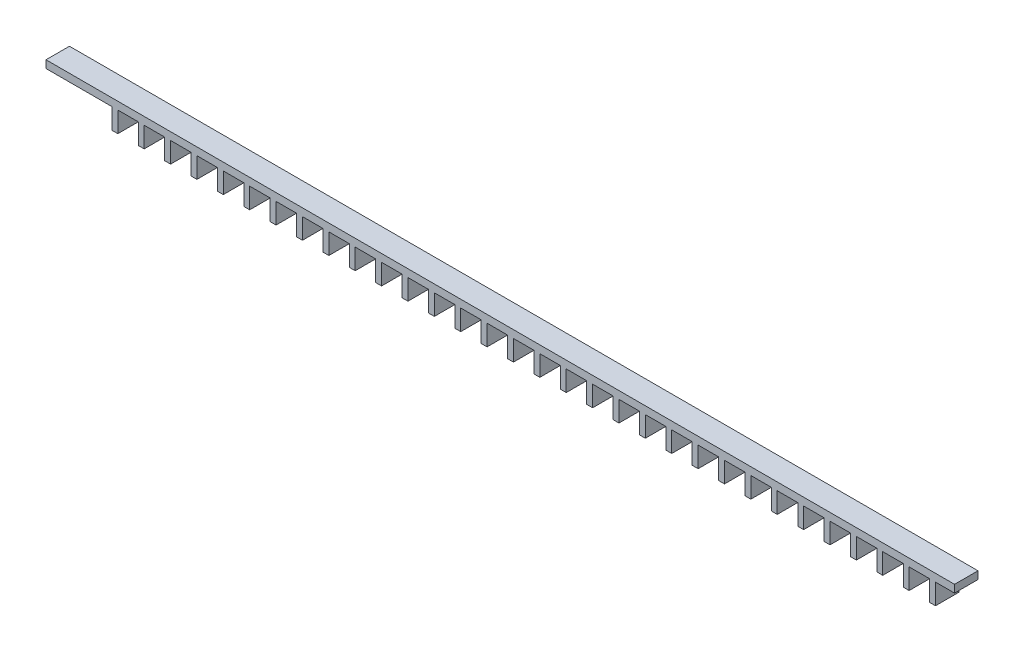
from build123d import *

# Parameters (mm, degrees)
SKETCH_1_W          = 1550
SKETCH_1_H          = 40
EXTRUDE_1_DEPTH     = 48
SKETCH_2_W          = 35
SKETCH_2_H          = 35
CUT_EXTRUDE_1_DEPTH = 778.514630087
SKETCH_6_W          = 35
SKETCH_6_H          = 35
CUT_EXTRUDE_5_DEPTH = 778.514630087
SKETCH_7_W          = 110
SKETCH_7_H          = 61.445783933
SKETCH_7_W_2        = 90
SKETCH_7_H_2        = 84.634966513
CUT_EXTRUDE_6_DEPTH = 778.514630087
SKETCH_8_W          = 40
SKETCH_8_H          = 13
EXTRUDE_2_DEPTH     = 10
SKETCH_9_W          = 40
SKETCH_9_H          = 13
CUT_EXTRUDE_7_DEPTH = 10
SKETCH_10_W         = 40
SKETCH_10_H         = 35
EXTRUDE_3_DEPTH     = 5
SKETCH_11_W         = 40
SKETCH_11_H         = 35
EXTRUDE_4_DEPTH     = 5
MOVE_FACE_1_BY      = 22.5
MOVE_FACE_1_2_BY    = 22.5
SKETCH_12_W         = 10
SKETCH_12_H         = 35
EXTRUDE_5_DEPTH     = 40
MOVE_FACE_2_BY      = 40
MOVE_FACE_2_2_BY    = 40


with BuildPart() as part:
    # 草图1 → 凸台-拉伸1 (new body)
    with BuildSketch(Plane(origin=(0, 0, 0), x_dir=(1, 0, 0), z_dir=(0, 1, 0))):
        Rectangle(SKETCH_1_W, SKETCH_1_H)
    extrude(amount=EXTRUDE_1_DEPTH)

    # 草图2 → 切除-拉伸1 (cut, through all)
    with BuildSketch(Plane.XY.offset(20)):
        with Locations((-752.5, 17.5)):
            Rectangle(SKETCH_2_W, SKETCH_2_H)
        with Locations((-707.5, 17.5)):
            Rectangle(SKETCH_2_W, SKETCH_2_H)
        with Locations((-662.5, 17.5)):
            Rectangle(SKETCH_2_W, SKETCH_2_H)
        with Locations((-617.5, 17.5)):
            Rectangle(SKETCH_2_W, SKETCH_2_H)
        with Locations((-572.5, 17.5)):
            Rectangle(SKETCH_2_W, SKETCH_2_H)
        with Locations((-527.5, 17.5)):
            Rectangle(SKETCH_2_W, SKETCH_2_H)
        with Locations((-482.5, 17.5)):
            Rectangle(SKETCH_2_W, SKETCH_2_H)
        with Locations((-437.5, 17.5)):
            Rectangle(SKETCH_2_W, SKETCH_2_H)
        with Locations((-392.5, 17.5)):
            Rectangle(SKETCH_2_W, SKETCH_2_H)
        with Locations((-347.5, 17.5)):
            Rectangle(SKETCH_2_W, SKETCH_2_H)
        with Locations((-302.5, 17.5)):
            Rectangle(SKETCH_2_W, SKETCH_2_H)
        with Locations((-257.5, 17.5)):
            Rectangle(SKETCH_2_W, SKETCH_2_H)
    extrude(amount=-CUT_EXTRUDE_1_DEPTH, mode=Mode.SUBTRACT)

    # 草图6 → 切除-拉伸5 (cut, through all)
    with BuildSketch(Plane.XY.offset(20)):
        with Locations((-212.5, 17.5)):
            Rectangle(SKETCH_6_W, SKETCH_6_H)
        with Locations((-77.5, 17.5)):
            Rectangle(SKETCH_6_W, SKETCH_6_H)
        with Locations((-167.5, 17.5)):
            Rectangle(SKETCH_6_W, SKETCH_6_H)
        with Locations((-122.5, 17.5)):
            Rectangle(SKETCH_6_W, SKETCH_6_H)
        with Locations((-32.5, 17.5)):
            Rectangle(SKETCH_6_W, SKETCH_6_H)
        with Locations((12.5, 17.5)):
            Rectangle(SKETCH_6_W, SKETCH_6_H)
        with Locations((57.5, 17.5)):
            Rectangle(SKETCH_6_W, SKETCH_6_H)
        with Locations((102.5, 17.5)):
            Rectangle(SKETCH_6_W, SKETCH_6_H)
        with Locations((147.5, 17.5)):
            Rectangle(SKETCH_6_W, SKETCH_6_H)
        with Locations((192.5, 17.5)):
            Rectangle(SKETCH_6_W, SKETCH_6_H)
        with Locations((237.5, 17.5)):
            Rectangle(SKETCH_6_W, SKETCH_6_H)
        with Locations((282.5, 17.5)):
            Rectangle(SKETCH_6_W, SKETCH_6_H)
        with Locations((327.5, 17.5)):
            Rectangle(SKETCH_6_W, SKETCH_6_H)
        with Locations((372.5, 17.5)):
            Rectangle(SKETCH_6_W, SKETCH_6_H)
        with Locations((417.5, 17.5)):
            Rectangle(SKETCH_6_W, SKETCH_6_H)
        with Locations((462.5, 17.5)):
            Rectangle(SKETCH_6_W, SKETCH_6_H)
        with Locations((507.5, 17.5)):
            Rectangle(SKETCH_6_W, SKETCH_6_H)
        with Locations((552.5, 17.5)):
            Rectangle(SKETCH_6_W, SKETCH_6_H)
        with Locations((597.5, 17.5)):
            Rectangle(SKETCH_6_W, SKETCH_6_H)
        with Locations((642.5, 17.5)):
            Rectangle(SKETCH_6_W, SKETCH_6_H)
        with Locations((687.5, 17.5)):
            Rectangle(SKETCH_6_W, SKETCH_6_H)
        with Locations((732.5, 17.5)):
            Rectangle(SKETCH_6_W, SKETCH_6_H)
    extrude(amount=-CUT_EXTRUDE_5_DEPTH, mode=Mode.SUBTRACT)

    # 草图7 → 切除-拉伸6 (cut, through all)
    with BuildSketch(Plane(origin=(0, 0, -20), x_dir=(-1, 0, 0), z_dir=(0, 0, -1))):
        with Locations((-720, 4.277108033)):
            Rectangle(SKETCH_7_W, SKETCH_7_H)
        with Locations((730, -7.317483257)):
            Rectangle(SKETCH_7_W_2, SKETCH_7_H_2)
    extrude(amount=-CUT_EXTRUDE_6_DEPTH, mode=Mode.SUBTRACT)

    # 草图8 → 凸台-拉伸2 (add)
    with BuildSketch(Plane.ZY.offset(775)):
        with Locations((0, 41.5)):
            Rectangle(SKETCH_8_W, SKETCH_8_H)
    extrude(amount=EXTRUDE_2_DEPTH)

    # 草图9 → 切除-拉伸7 (cut)
    with BuildSketch(Plane(origin=(775, 0, 0), x_dir=(0, 0, -1), z_dir=(1, 0, 0))):
        with Locations((0, 41.5)):
            Rectangle(SKETCH_9_W, SKETCH_9_H)
    extrude(amount=-CUT_EXTRUDE_7_DEPTH, mode=Mode.SUBTRACT)

    # 草图10 → 凸台-拉伸3 (add)
    with BuildSketch(Plane(origin=(665, 0, 0), x_dir=(0, 0, -1), z_dir=(1, 0, 0))):
        with Locations((0, 17.5)):
            Rectangle(SKETCH_10_W, SKETCH_10_H)
    extrude(amount=EXTRUDE_3_DEPTH)

    # 草图11 → 凸台-拉伸4 (add)
    with BuildSketch(Plane.ZY.offset(685)):
        with Locations((0, 17.5)):
            Rectangle(SKETCH_11_W, SKETCH_11_H)
    extrude(amount=EXTRUDE_4_DEPTH)

    # Move Face 1: a face moved outward by 22.5
    extrude(part.faces().sort_by_distance((-785, 41.5, 0))[0], amount=MOVE_FACE_1_BY, dir=(-1, 0, 0))

    # Move Face 1 2: a face moved inward by 22.5
    extrude(part.faces().sort_by_distance((765, 41.5, 0))[0], amount=MOVE_FACE_1_2_BY, dir=(-1, 0, 0), mode=Mode.SUBTRACT)

    # 草图12 → 凸台-拉伸5 (add)
    with BuildSketch(Plane.XY.offset(20)):
        with Locations((-730, 17.5)):
            Rectangle(SKETCH_12_W, SKETCH_12_H)
    extrude(amount=-EXTRUDE_5_DEPTH)

    # Move Face 2: a face moved outward by 40.0
    extrude(part.faces().sort_by_distance((-807.5, 41.5, 0))[0], amount=MOVE_FACE_2_BY, dir=(-1, 0, 0))

    # Move Face 2 2: a face moved inward by 40.0
    extrude(part.faces().sort_by_distance((742.5, 41.5, 0))[0], amount=MOVE_FACE_2_2_BY, dir=(-1, 0, 0), mode=Mode.SUBTRACT)


solid = part.part
